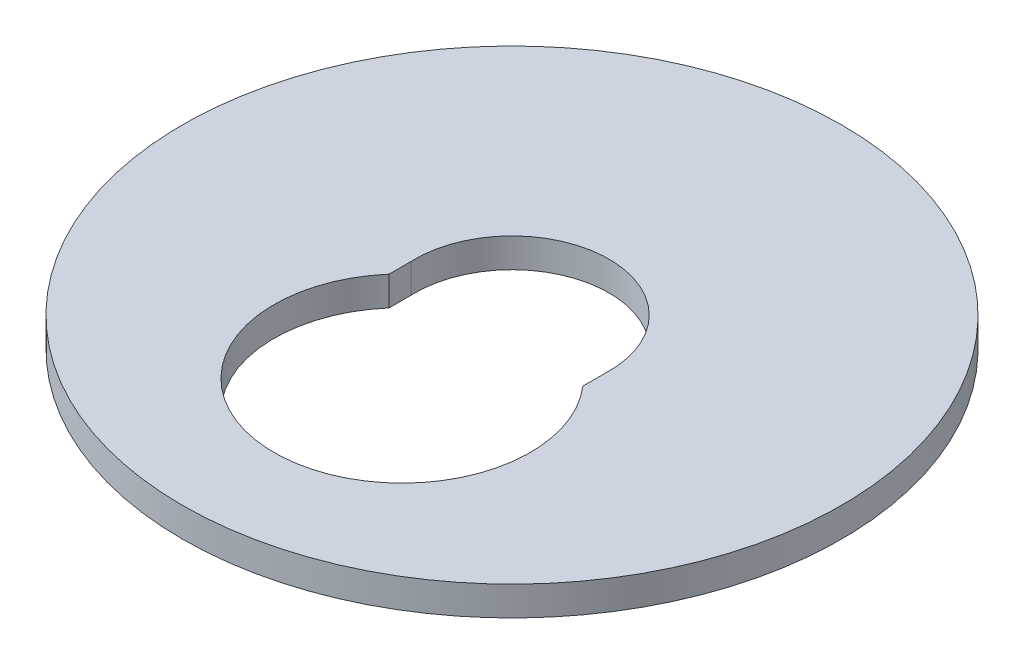
SolidWorks part; units mm, degrees
ref_plane "前视基准面" through (0, 0, 0) normal (0, 0, 1) x (1, 0, 0)
ref_plane "上视基准面" through (0, 0, 0) normal (0, 1, 0) x (1, 0, 0)
ref_plane "右视基准面" through (0, 0, 0) normal (1, 0, 0) x (0, 0, -1)
sketch "草图1" plane through (0, 0, 0) normal (0, 1, 0) x (1, 0, 0)
  circle A0 centre (0, 0) radius 13.25
  circle A1 centre (0, 0) radius 45
  dimension "D1" = 26.5
  dimension "D2" = 90
extrude "凸台-拉伸1" add sketch "草图1" along normal mid plane 4
sketch "草图2" plane through (0, -2, 0) normal (0, -1, 0) x (1, 0, 0)
  line L0 (-13.2384, 0.5547) -> (-13.2384, 3.5547)
  line L1 (13.2384, 0.5547) -> (13.2384, 3.5547)
  line L2 (-13.2384, 0.5547) -> (13.2384, 0.5547)
  circle A0 centre (0, 0) radius 13.25 construction
  arc A1 (13.2384, 3.5547) -> (-13.2384, 3.5547) centre (0, 15) ccw
  point P7 (-12.9265, 2.984)
  dimension "D1" = 35
  dimension "D2" = 3
  dimension "D3" = 15
extrude "切除-拉伸1" cut sketch "草图2" against normal up to next
